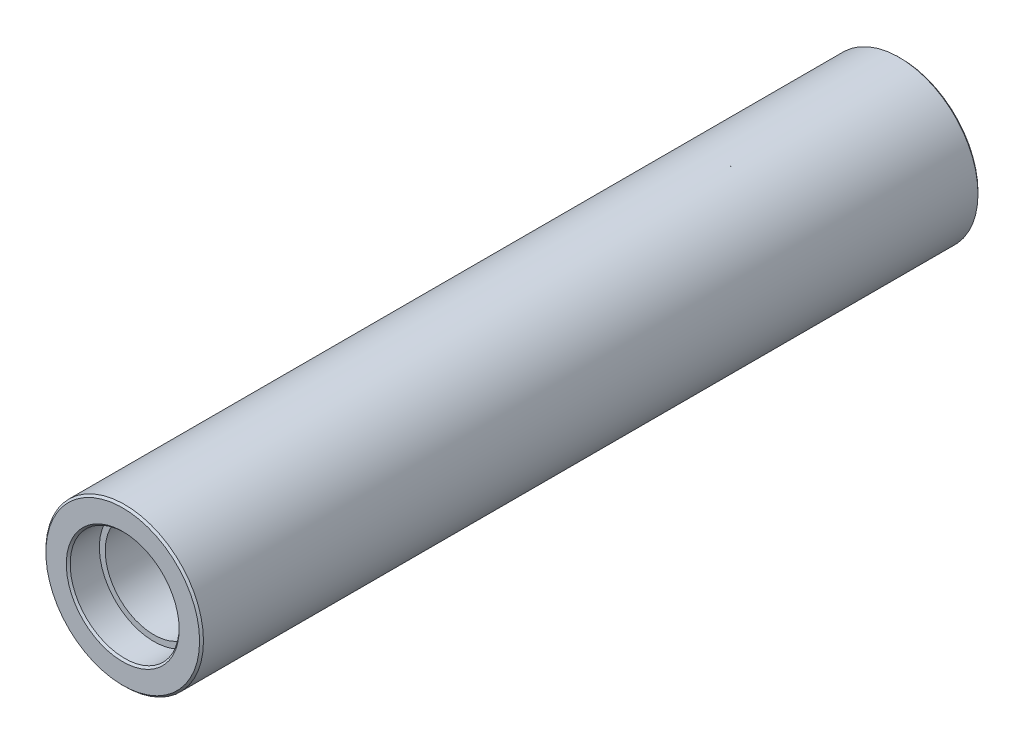
from build123d import *

# Parameters (mm, degrees)
SKETCH_1_R          = 20.25
EXTRUDE_1_DEPTH     = 100
SKETCH_2_R          = 14
CUT_EXTRUDE_1_DEPTH = 8
SKETCH_3_R          = 12.5
CUT_EXTRUDE_2_DEPTH = 195.12399388
CHAMFER_1_SIZE      = 0.5


with BuildPart() as part:
    # 草图1 → 凸台-拉伸1 (new, symmetric)
    with BuildSketch(Plane.XY):
        Circle(SKETCH_1_R)
    extrude(amount=EXTRUDE_1_DEPTH, both=True)

    # 草图2 → 切除-拉伸1 (cut)
    with BuildSketch(Plane.XY.offset(100)):
        Circle(SKETCH_2_R)
    cut_extrude_1 = extrude(amount=-CUT_EXTRUDE_1_DEPTH, mode=Mode.SUBTRACT)

    # 镜向1: 切除-拉伸1 across plane
    add(cut_extrude_1.mirror(Plane.XY), mode=Mode.SUBTRACT)

    # 草图3 → 切除-拉伸2 (cut, through all)
    with BuildSketch(Plane.XY.offset(92)):
        Circle(SKETCH_3_R)
    extrude(amount=-CUT_EXTRUDE_2_DEPTH, mode=Mode.SUBTRACT)

    # 倒角1
    chamfer_1_edges = [part.edges().sort_by_distance(p)[0] for p in [
        (-14, 0, -100),
        (-20.25, 0, -100),
        (-20.25, 0, 100),
        (-14, 0, 100),
    ]]
    chamfer(chamfer_1_edges, length=CHAMFER_1_SIZE)


solid = part.part
